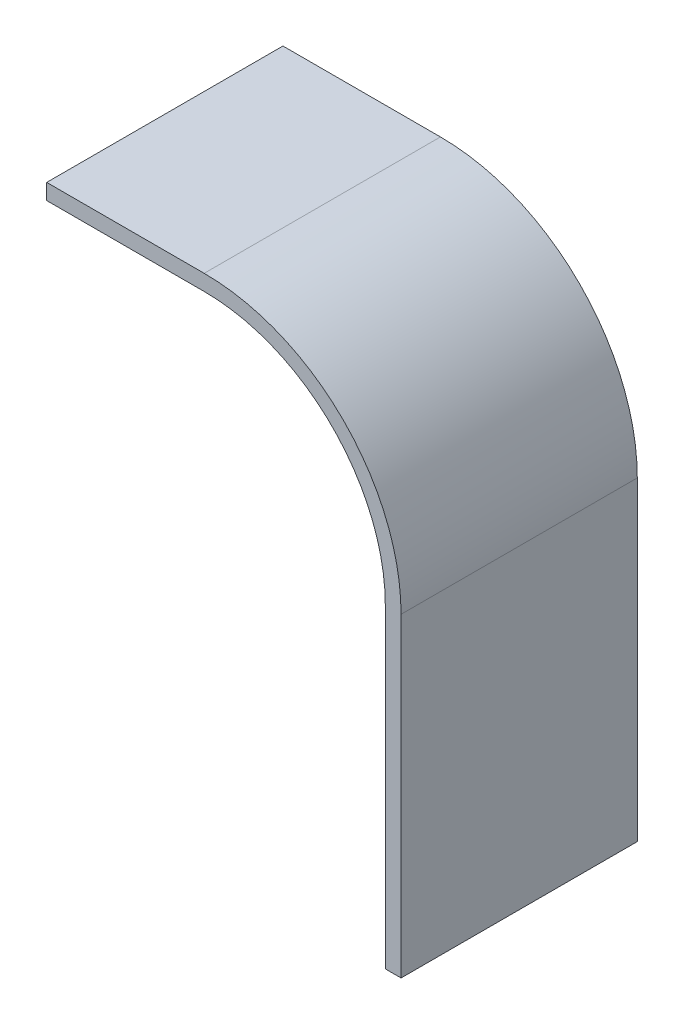
from build123d import *

# Parameters (mm, degrees)
EXTRUDE_THIN1_DEPTH = 2
BOSS_EXTRUDE1_DEPTH = 28
CUT_EXTRUDE1_DEPTH  = 28


with BuildPart() as part:
    # Sketch1 → Extrude-Thin1 (new body)
    with BuildSketch(Plane.XY):
        with BuildLine():
            Line((0, 0), (0, 40))
            ThreePointArc((0, 40), (-2.928932188, 47.071067812), (-10, 50))
            Line((-10, 50), (-30, 50))
            Line((-30, 50), (-30, 65))
            Line((-30, 65), (-10, 65))
            ThreePointArc((-10, 65), (7.67766953, 57.67766953), (15, 40))
            Line((15, 40), (15, 0))
            Line((15, 0), (0, 0))
        make_face()
    extrude(amount=EXTRUDE_THIN1_DEPTH)

    # Sketch2 → Boss-Extrude1 (add)
    with BuildSketch(Plane.XY.offset(2)):
        with BuildLine():
            Line((13, 0), (13, 40))
            ThreePointArc((13, 40), (6.263455967, 56.263455967), (-10, 63))
            Line((-10, 63), (-30, 63))
            Line((-30, 63), (-30, 65))
            Line((-30, 65), (-10, 65))
            ThreePointArc((-10, 65), (7.67766953, 57.67766953), (15, 40))
            Line((15, 40), (15, 0))
            Line((15, 0), (13, 0))
        make_face()
    extrude(amount=BOSS_EXTRUDE1_DEPTH)

    # Sketch3 → Cut-Extrude1 (cut)
    with BuildSketch(Plane.XY.offset(2)):
        with BuildLine():
            Line((-19.283890524, 59.176308794), (-19.283890524, 52.835918308))
            ThreePointArc((-19.283890524, 52.835918308), (-21.035277496, 51.084531336), (-22.786664469, 52.835918308))
            Line((-22.786664469, 52.835918308), (-22.786664469, 59.176308794))
            ThreePointArc((-22.786664469, 59.176308794), (-21.035277496, 60.927695767), (-19.283890524, 59.176308794))
        make_face()
        with BuildLine():
            Line((3.842402099, 13.695706596), (8.588468352, 13.695706596))
            ThreePointArc((8.588468352, 13.695706596), (10.164668971, 12.119505978), (8.588468352, 10.543305359))
            Line((8.588468352, 10.543305359), (3.842402099, 10.543305359))
            ThreePointArc((3.842402099, 10.543305359), (2.26620148, 12.119505978), (3.842402099, 13.695706596))
        make_face()
        with BuildLine():
            Line((3.842402099, 37.707268764), (8.588468352, 37.707268764))
            ThreePointArc((8.588468352, 37.707268764), (10.388432438, 35.907304678), (8.588468352, 34.107340593))
            Line((8.588468352, 34.107340593), (3.842402099, 34.107340593))
            ThreePointArc((3.842402099, 34.107340593), (2.042438013, 35.907304678), (3.842402099, 37.707268764))
        make_face()
    extrude(amount=-CUT_EXTRUDE1_DEPTH, mode=Mode.SUBTRACT)


solid = part.part
